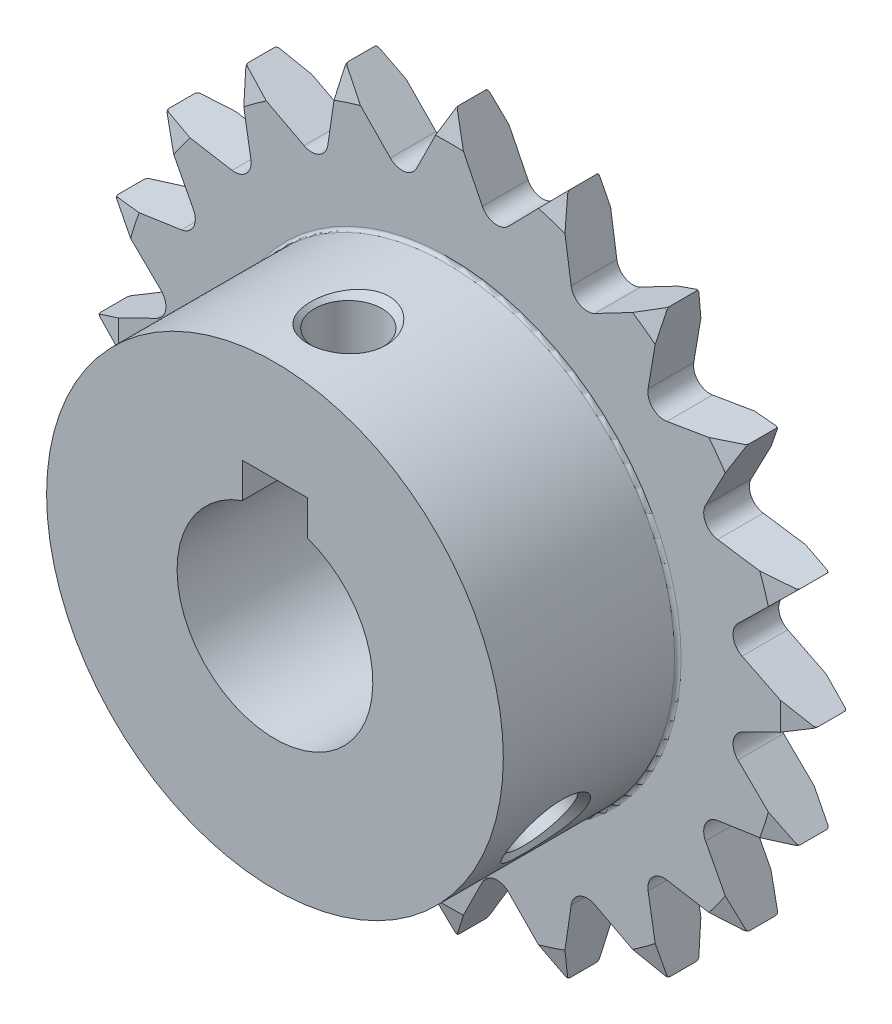
from build123d import *

# Parameters (mm, degrees)
SKETCH_2_W               = 302.005499825
SKETCH_2_H               = 246.129864536
CUT_EXTRUDE_1_DEPTH      = 2.8
SKETCH_5_W               = 4
SKETCH_5_H               = 7.8
CUT_EXTRUDE_2_DEPTH      = 15
CUT_EXTRUDE_3_DEPTH      = 35.539832206
CUT_EXTRUDE_3_DEPTH_BACK = 35.539832206
SKETCH_6_W               = 29.085474913
SKETCH_6_H               = 1.5


with BuildPart() as part:
    # 草图1 → 旋转1 (revolve)
    with BuildSketch(Plane(origin=(0, 0, 0), x_dir=(0, 0, -1), z_dir=(1, 0, 0)), mode=Mode.PRIVATE) as revolve_1_sk:
        with BuildLine():
            Line((-15, 6.2), (-14.8, 6))
            Line((-14.8, 6), (-0.2, 6))
            Line((-0.2, 6), (0, 6.2))
            Line((0, 6.2), (0, 20.295))
            Line((0, 20.295), (-0.417133605, 21.851763809))
            ThreePointArc((-0.417133605, 21.851763809), (-0.488566485, 21.958670668), (-0.610318771, 22))
            Line((-0.610318771, 22), (-2.189681229, 22))
            ThreePointArc((-2.189681229, 22), (-2.311433515, 21.958670668), (-2.382866395, 21.851763809))
            Line((-2.382866395, 21.851763809), (-2.8, 20.295))
            Line((-2.8, 20.295), (-2.8, 14.2))
            ThreePointArc((-2.8, 14.2), (-2.858578644, 14.058578644), (-3, 14))
            Line((-3, 14), (-14.8, 14))
            Line((-14.8, 14), (-15, 13.8))
            Line((-15, 13.8), (-15, 6.2))
        make_face()
    revolve(revolve_1_sk.sketch.rotate(Axis((0, 0, 0), (0, 0, 1)), 270), axis=Axis((0, 0, 0), (0, 0, 1)))

    # 草图2 → 切除-拉伸1 (cut)
    with BuildSketch(Plane.XY):
        with Locations((0.692673165, 3.694256879)):
            Rectangle(SKETCH_2_W, SKETCH_2_H)
        with BuildLine():
            Line((-22, 0), (-17.937956487, -2.01572466))
            ThreePointArc((-17.937956487, -2.01572466), (-17.394781022, -2.755062657), (-17.682903582, -3.626065326))
            Line((-17.682903582, -3.626065326), (-20.923243358, -6.798373876))
            Line((-20.923243358, -6.798373876), (-16.43711723, -7.460201472))
            ThreePointArc((-16.43711723, -7.460201472), (-15.692058659, -7.995503242), (-15.69692487, -8.912910774))
            Line((-15.69692487, -8.912910774), (-17.798373876, -12.93127555))
            Line((-17.798373876, -12.93127555), (-13.327298415, -12.174421785))
            ThreePointArc((-13.327298415, -12.174421785), (-12.453288261, -12.453288261), (-12.174421785, -13.327298415))
            Line((-12.174421785, -13.327298415), (-12.93127555, -17.798373876))
            Line((-12.93127555, -17.798373876), (-8.912910774, -15.69692487))
            ThreePointArc((-8.912910774, -15.69692487), (-7.995503242, -15.692058659), (-7.460201472, -16.43711723))
            Line((-7.460201472, -16.43711723), (-6.798373876, -20.923243358))
            Line((-6.798373876, -20.923243358), (-3.626065326, -17.682903582))
            ThreePointArc((-3.626065326, -17.682903582), (-2.755062657, -17.394781022), (-2.01572466, -17.937956487))
            Line((-2.01572466, -17.937956487), (0, -22))
            Line((0, -22), (2.01572466, -17.937956487))
            ThreePointArc((2.01572466, -17.937956487), (2.755062657, -17.394781022), (3.626065326, -17.682903582))
            Line((3.626065326, -17.682903582), (6.798373876, -20.923243358))
            Line((6.798373876, -20.923243358), (7.460201472, -16.43711723))
            ThreePointArc((7.460201472, -16.43711723), (7.995503242, -15.692058659), (8.912910774, -15.69692487))
            Line((8.912910774, -15.69692487), (12.93127555, -17.798373876))
            Line((12.93127555, -17.798373876), (12.174421785, -13.327298415))
            ThreePointArc((12.174421785, -13.327298415), (12.453288261, -12.453288261), (13.327298415, -12.174421785))
            Line((13.327298415, -12.174421785), (17.798373876, -12.93127555))
            Line((17.798373876, -12.93127555), (15.69692487, -8.912910774))
            ThreePointArc((15.69692487, -8.912910774), (15.692058659, -7.995503242), (16.43711723, -7.460201472))
            Line((16.43711723, -7.460201472), (20.923243358, -6.798373876))
            Line((20.923243358, -6.798373876), (17.682903582, -3.626065326))
            ThreePointArc((17.682903582, -3.626065326), (17.394781022, -2.755062657), (17.937956487, -2.01572466))
            Line((17.937956487, -2.01572466), (22, 0))
            Line((22, 0), (17.937956487, 2.01572466))
            ThreePointArc((17.937956487, 2.01572466), (17.394781022, 2.755062657), (17.682903582, 3.626065326))
            Line((17.682903582, 3.626065326), (20.923243358, 6.798373876))
            Line((20.923243358, 6.798373876), (16.43711723, 7.460201472))
            ThreePointArc((16.43711723, 7.460201472), (15.692058659, 7.995503242), (15.69692487, 8.912910774))
            Line((15.69692487, 8.912910774), (17.798373876, 12.93127555))
            Line((17.798373876, 12.93127555), (13.327298415, 12.174421785))
            ThreePointArc((13.327298415, 12.174421785), (12.453288261, 12.453288261), (12.174421785, 13.327298415))
            Line((12.174421785, 13.327298415), (12.93127555, 17.798373876))
            Line((12.93127555, 17.798373876), (8.912910774, 15.69692487))
            ThreePointArc((8.912910774, 15.69692487), (7.995503242, 15.692058659), (7.460201472, 16.43711723))
            Line((7.460201472, 16.43711723), (6.798373876, 20.923243358))
            Line((6.798373876, 20.923243358), (3.626065326, 17.682903582))
            ThreePointArc((3.626065326, 17.682903582), (2.755062657, 17.394781022), (2.01572466, 17.937956487))
            Line((2.01572466, 17.937956487), (0, 22))
            Line((0, 22), (-2.01572466, 17.937956487))
            ThreePointArc((-2.01572466, 17.937956487), (-2.755062657, 17.394781022), (-3.626065326, 17.682903582))
            Line((-3.626065326, 17.682903582), (-6.798373876, 20.923243358))
            Line((-6.798373876, 20.923243358), (-7.460201472, 16.43711723))
            ThreePointArc((-7.460201472, 16.43711723), (-7.995503242, 15.692058659), (-8.912910774, 15.69692487))
            Line((-8.912910774, 15.69692487), (-12.93127555, 17.798373876))
            Line((-12.93127555, 17.798373876), (-12.174421785, 13.327298415))
            ThreePointArc((-12.174421785, 13.327298415), (-12.453288261, 12.453288261), (-13.327298415, 12.174421785))
            Line((-13.327298415, 12.174421785), (-17.798373876, 12.93127555))
            Line((-17.798373876, 12.93127555), (-15.69692487, 8.912910774))
            ThreePointArc((-15.69692487, 8.912910774), (-15.692058659, 7.995503242), (-16.43711723, 7.460201472))
            Line((-16.43711723, 7.460201472), (-20.923243358, 6.798373876))
            Line((-20.923243358, 6.798373876), (-17.682903582, 3.626065326))
            ThreePointArc((-17.682903582, 3.626065326), (-17.394781022, 2.755062657), (-17.937956487, 2.01572466))
            Line((-17.937956487, 2.01572466), (-22, 0))
        make_face(mode=Mode.SUBTRACT)
    extrude(amount=CUT_EXTRUDE_1_DEPTH, mode=Mode.SUBTRACT)

    # 草图3 → 切除-旋转1 (revolve, cut)
    with BuildSketch(Plane.XY.offset(9), mode=Mode.PRIVATE) as cut_revolve_1_sk:
        Polygon((0, 1.8), (-2.5, 1.8), (-2.5, 7.8), (-2.067, 8.233), (-2.067, 13.567), (-2.5, 14), (-2.5, 20), (0, 20), align=None)
    revolve(cut_revolve_1_sk.sketch.rotate(Axis((0, 14, 9), (0, -1, 0)), 180), axis=Axis((0, 14, 9), (0, -1, 0)), mode=Mode.SUBTRACT)

    # 草图4 → 切除-旋转2 (revolve, cut)
    with BuildSketch(Plane.XY.offset(9), mode=Mode.PRIVATE) as cut_revolve_2_sk:
        Polygon((0, 0), (1.25, 2.165063509), (6.446152423, -0.834936491), (6.604641423, -1.42642549), (12.782866653, -4.99342549), (13.374355653, -4.834936491), (18.570508076, -7.834936491), (17.320508076, -10), align=None)
    revolve(cut_revolve_2_sk.sketch.rotate(Axis((12.124355653, -7, 9), (-0.8660254037844384, 0.5000000000000007, 0)), 180), axis=Axis((12.124355653, -7, 9), (-0.8660254037844384, 0.5000000000000007, 0)), mode=Mode.SUBTRACT)

    # 草图5 → 切除-拉伸2 (cut)
    with BuildSketch(Plane.XY):
        with Locations((0, 3.9)):
            Rectangle(SKETCH_5_W, SKETCH_5_H)
    extrude(amount=CUT_EXTRUDE_2_DEPTH, mode=Mode.SUBTRACT)

    # 草图6 → 切除-拉伸3 (cut, two sides: drawn at the far end of the back side and taken through both)
    with BuildSketch(Plane(origin=(0, 0, 0), x_dir=(1, 0, 0), z_dir=(0, 1, 0)).offset(-CUT_EXTRUDE_3_DEPTH_BACK)):
        with Locations((0.142559915, -14.25)):
            Rectangle(SKETCH_6_W, SKETCH_6_H)
    extrude(amount=CUT_EXTRUDE_3_DEPTH + CUT_EXTRUDE_3_DEPTH_BACK, mode=Mode.SUBTRACT)


solid = part.part
